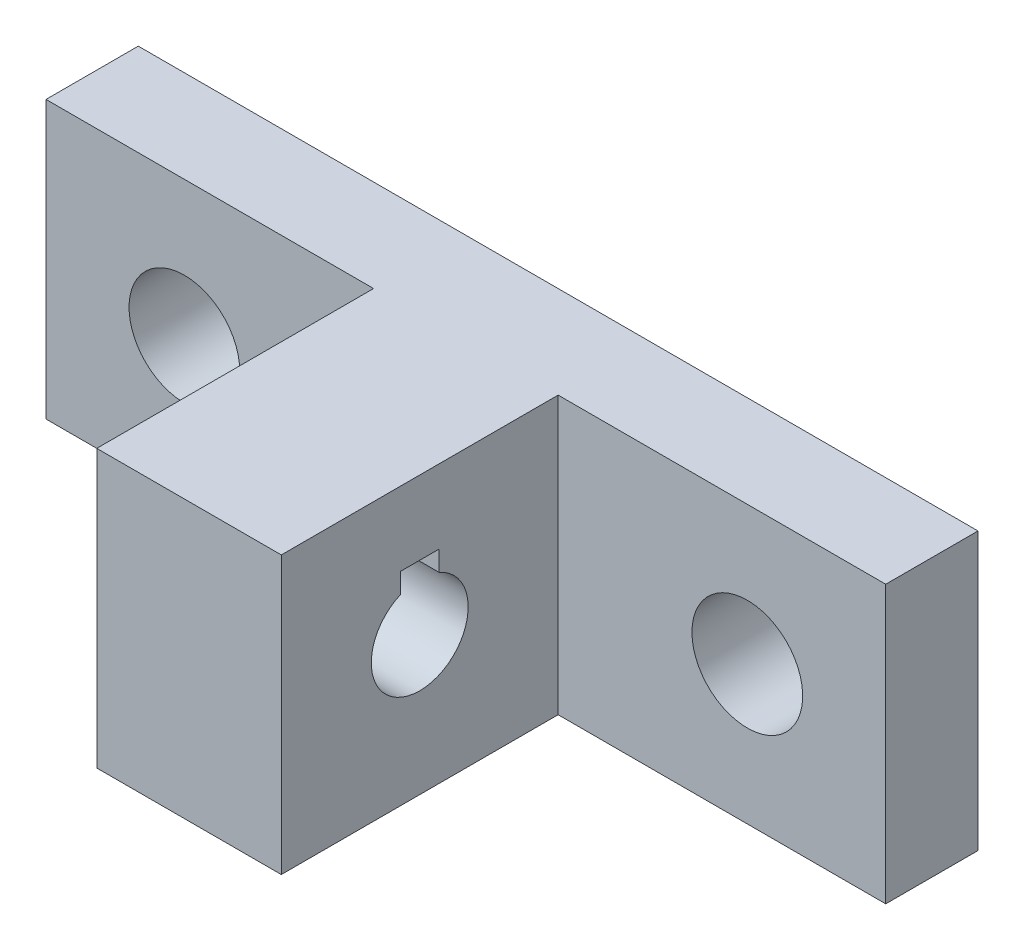
SolidWorks part; units mm, degrees
ref_plane "Front Plane" through (0, 0, 0) normal (0, 0, 1) x (1, 0, 0)
ref_plane "Top Plane" through (0, 0, 0) normal (0, 1, 0) x (1, 0, 0)
ref_plane "Right Plane" through (0, 0, 0) normal (1, 0, 0) x (0, 0, -1)
sketch "Sketch1" plane through (0, 0, 0) normal (0, 0, 1) x (1, 0, 0)
  line L1 (-45.5, -15) -> (45.5, -15)
  line L2 (-45.5, -15) -> (-45.5, 15)
  line L3 (-45.5, 15) -> (45.5, 15)
  line L4 (45.5, -15) -> (45.5, 15)
  line L5 (-45.5, -15) -> (45.5, 15) construction
  line L6 (-45.5, 15) -> (45.5, -15) construction
  point P0 (0, 0)
  dimension "D1" = 91
  dimension "D2" = 30
extrude "Boss-Extrude1" add sketch "Sketch1" along normal blind 10
sketch "Sketch2" plane through (0, 0, 10) normal (0, 0, 1) x (1, 0, 0)
  line L0 (45.5, 15) -> (-45.5, 15) construction
  line L1 (-10, -15) -> (10, -15)
  line L2 (-10, -15) -> (-10, 15)
  line L3 (-10, 15) -> (10, 15)
  line L4 (10, -15) -> (10, 15)
  line L5 (-10, -15) -> (10, 15) construction
  line L6 (-10, 15) -> (10, -15) construction
  point P0 (0, 0)
  dimension "D1" = 20
extrude "Boss-Extrude2" add sketch "Sketch2" along normal blind 30
sketch "Sketch4" plane through (-10, 0, 0) normal (-1, 0, 0) x (0, 0, 1)
  line L0 (40, 0) -> (10, 0) construction
  line L1 (40, 15) -> (40, -15) construction
  line L2 (10, 15) -> (10, -15) construction
  line L7 (27.1, 7) -> (22.9, 7)
  line L8 (27.1, 7) -> (27.1, 4.8117)
  line L9 (22.9, 7) -> (22.9, 4.8117)
  arc A0 (22.9, 4.8117) -> (27.1, 4.8117) centre (25, 0) ccw
  dimension "D1" = 10.5
  dimension "D2" = 4.2
  dimension "D3" = 7
extrude "Cut-Extrude1" cut sketch "Sketch4" against normal blind 30
sketch "Sketch5" plane through (0, 0, 10) normal (0, 0, 1) x (1, 0, 0)
  line L0 (-30.5, 0) -> (30.5, 0) construction
  line L1 (0, 15) -> (0, -2.4075) construction
  line L2 (10, 15) -> (-10, 15) construction
  circle A0 centre (-30.5, 0) radius 6
  circle A1 centre (30.5, 0) radius 6
  point P4 (0, 0)
  dimension "D2" = 12
  dimension "D1" = 61
extrude "Cut-Extrude2" cut sketch "Sketch5" against normal blind 30
